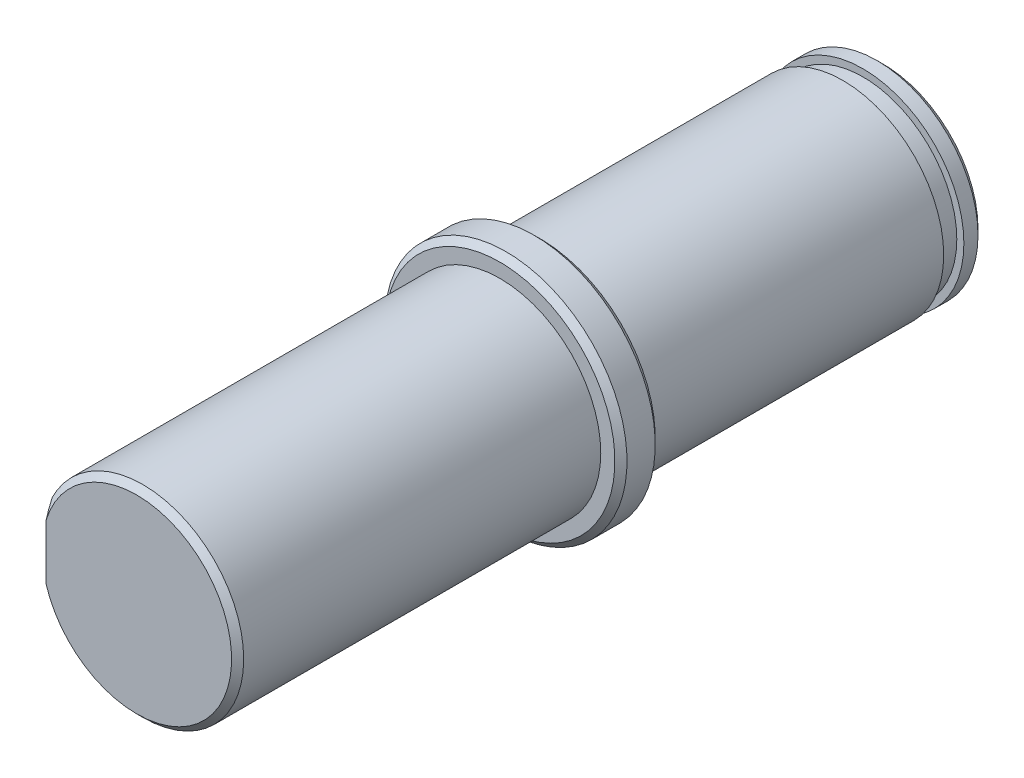
from build123d import *

# Parameters (mm, degrees)
SKETCH1_R               = 5
BOSS_EXTRUDE1_DEPTH     = 18
SKETCH2_R               = 6
BOSS_EXTRUDE2_DEPTH     = 2
BOSS_EXTRUDE3_START     = 17
SKETCH3_R               = 5
BOSS_EXTRUDE3_DEPTH     = 17
SKETCH4_W               = 1.979153599
SKETCH4_H               = 1
CUT_EXTRUDE1_DEPTH      = 10
CUT_EXTRUDE1_DEPTH_BACK = 10
SKETCH5_W               = 5.566789872
SKETCH5_H               = 10
CHAMFER1_SIZE           = 0.3


with BuildPart() as part:
    # Sketch1 → Boss-Extrude1 (new body)
    with BuildSketch(Plane.XY):
        Circle(SKETCH1_R)
    extrude(amount=BOSS_EXTRUDE1_DEPTH)

    # Sketch2 → Boss-Extrude2 (add)
    with BuildSketch(Plane(origin=(0, 0, 0), x_dir=(-1, 0, 0), z_dir=(0, 0, -1))):
        Circle(SKETCH2_R)
    extrude(amount=BOSS_EXTRUDE2_DEPTH)

    # Sketch3 → Boss-Extrude3 (add)
    with BuildSketch(Plane(origin=(0, 0, -2), x_dir=(-1, 0, 0), z_dir=(0, 0, -1)).offset(BOSS_EXTRUDE3_START)):
        Circle(SKETCH3_R)
    extrude(amount=-BOSS_EXTRUDE3_DEPTH)

    # Sketch4 → Cut-Revolve1 (revolve, cut)
    with BuildSketch(Plane(origin=(0, 0, 0), x_dir=(1, 0, 0), z_dir=(0, 1, 0))):
        with Locations((-5.6395768, 17.5)):
            Rectangle(SKETCH4_W, SKETCH4_H)
    revolve(axis=Axis((0, 0, -19), (0, 0, 1)), mode=Mode.SUBTRACT)

    # Sketch5 → Cut-Extrude1 (cut, two sides: drawn at the far end of the back side and taken through both)
    with BuildSketch(Plane(origin=(0, 0, 0), x_dir=(1, 0, 0), z_dir=(0, 1, 0)).offset(-CUT_EXTRUDE1_DEPTH_BACK)):
        with Locations((-7.283394936, -13)):
            Rectangle(SKETCH5_W, SKETCH5_H)
    extrude(amount=CUT_EXTRUDE1_DEPTH + CUT_EXTRUDE1_DEPTH_BACK, mode=Mode.SUBTRACT)

    # Chamfer1
    chamfer1_edges = [part.edges().sort_by_distance(p)[0] for p in [
        (5, 0, -19),
        (1.118033989, -4.873397172, 18),
        (6, 0, 0),
        (6, 0, -2),
    ]]
    chamfer(chamfer1_edges, length=CHAMFER1_SIZE)


solid = part.part
